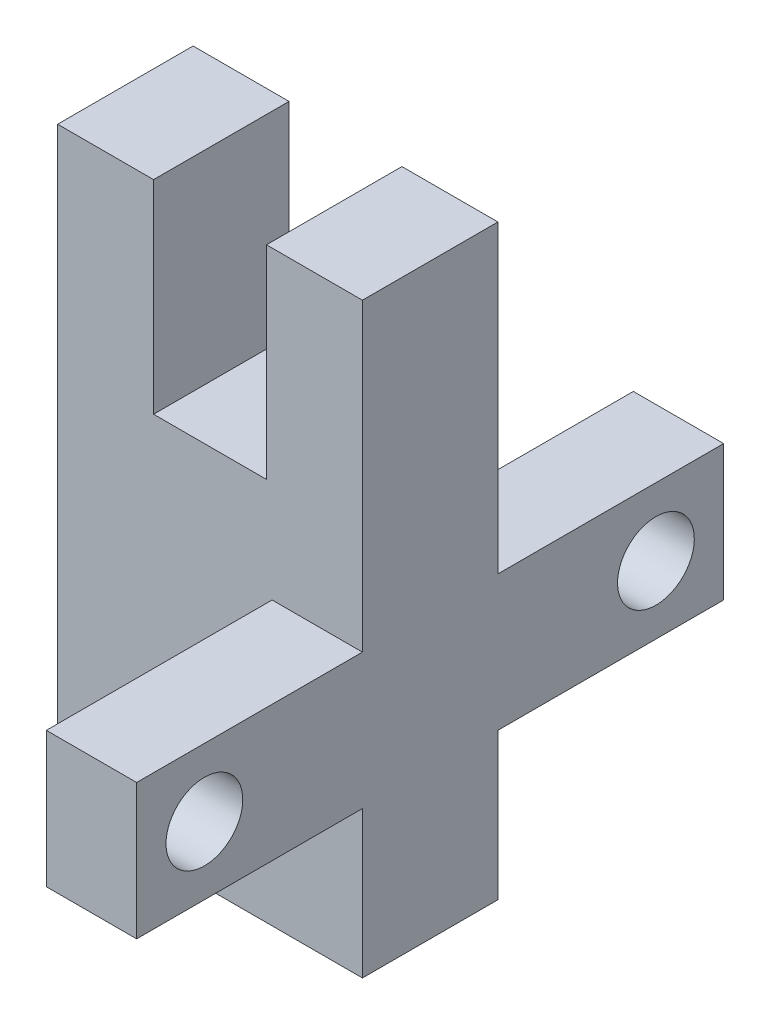
SolidWorks part; units mm, degrees
ref_plane "Front Plane" through (0, 0, 0) normal (0, 0, 1) x (1, 0, 0)
ref_plane "Top Plane" through (0, 0, 0) normal (0, 1, 0) x (1, 0, 0)
ref_plane "Right Plane" through (0, 0, 0) normal (1, 0, 0) x (0, 0, -1)
sketch "Sketch1" plane through (0, 0, 0) normal (0, 0, 1) x (1, 0, 0)
  line L0 (9.25, 0) -> (13.5, 0)
  line L1 (0, 0) -> (4.25, 0)
  line L2 (0, 0) -> (0, -26)
  line L3 (0, -26) -> (13.5, -26)
  line L4 (13.5, 0) -> (13.5, -26)
  line L6 (4.25, 0) -> (4.25, -9)
  line L7 (4.25, -9) -> (9.25, -9)
  line L8 (9.25, 0) -> (9.25, -9)
  dimension "D1" = 4.25
  dimension "D2" = 9
  dimension "D3" = 26
  dimension "D4" = 13.5
  dimension "D5" = 4.25
extrude "Boss-Extrude1" add sketch "Sketch1" along normal mid plane 6
sketch "Sketch2" plane through (13.5, 0, 0) normal (1, 0, 0) x (0, 0, -1)
  line L0 (-3, 0) -> (3, 0) construction
  line L1 (-13, -13.5) -> (13, -13.5)
  line L2 (-13, -13.5) -> (-13, -19.5)
  line L3 (-13, -19.5) -> (13, -19.5)
  line L4 (13, -13.5) -> (13, -19.5)
  circle A0 centre (-10, -16.5) radius 1.7
  circle A1 centre (10, -16.5) radius 1.7
  dimension "D6" = 3.4
  dimension "D1" = 10
  dimension "D2" = 10
  dimension "D3" = 26
  dimension "D4" = 13
  dimension "D5" = 6
  dimension "D7" = 16.5
  dimension "D8" = 3
extrude "Boss-Extrude2" add sketch "Sketch2" against normal blind 4
